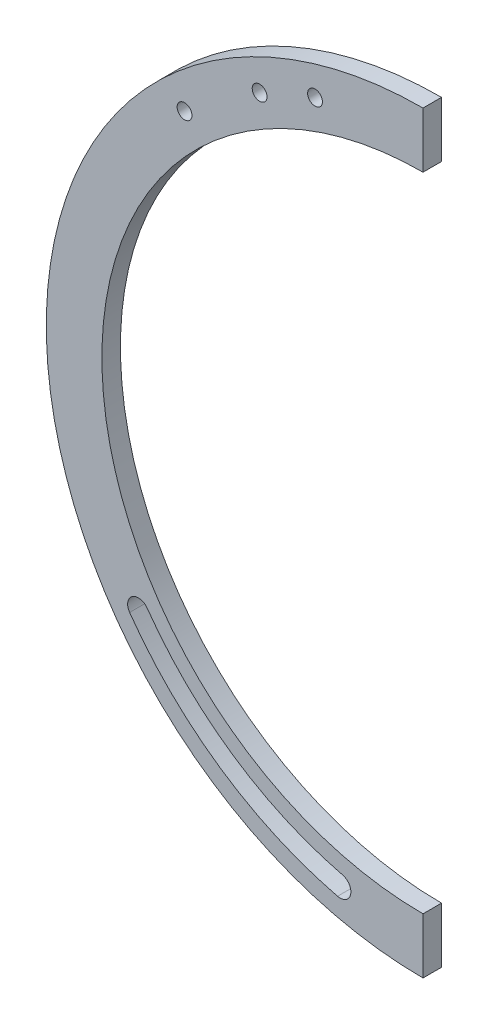
from build123d import *

# Parameters (mm, degrees)
SKETCH1_R               = 203.294925519
SKETCH1_R_2             = 173.294925519
BOSS_EXTRUDE1_DEPTH     = 10
CUT_EXTRUDE1_START      = -185
CUT_EXTRUDE1_DEPTH      = 185
CUT_EXTRUDE2_DEPTH      = 185
CUT_EXTRUDE3_DEPTH      = 484.877792972
CUT_EXTRUDE3_DEPTH_BACK = 484.877792972
SKETCH4_R               = 4


with BuildPart() as part:
    # Sketch1 → Boss-Extrude1 (new body)
    with BuildSketch(Plane.XY):
        with Locations((291.585214163, 182.730697222)):
            Circle(SKETCH1_R)
        with Locations((291.585214163, 182.730697222)):
            Circle(SKETCH1_R_2, mode=Mode.SUBTRACT)
    extrude(amount=-BOSS_EXTRUDE1_DEPTH)

    # Sketch2 → Cut-Extrude1 (cut)
    with BuildSketch(Plane(origin=(0, 0, -10), x_dir=(-1, 0, 0), z_dir=(0, 0, -1)).offset(CUT_EXTRUDE1_START)):
        with BuildLine():
            Line((-291.585214163, 9.435771703), (-291.585214163, -33.905509081))
            ThreePointArc((-291.585214163, -33.905509081), (-508.221420466, 182.730697222), (-291.585214163, 399.366903525))
            Line((-291.585214163, 399.366903525), (-291.585214163, 356.025622742))
            ThreePointArc((-291.585214163, 356.025622742), (-464.880139683, 182.730697222), (-291.585214163, 9.435771703))
        make_face()
    extrude(amount=CUT_EXTRUDE1_DEPTH, mode=Mode.SUBTRACT)

    # Sketch3 → Cut-Extrude2 (cut)
    with BuildSketch(Plane(origin=(0, 0, -10), x_dir=(-1, 0, 0), z_dir=(0, 0, -1))):
        with BuildLine():
            ThreePointArc((-245.463287057, -5.419646314), (-182.427275621, 22.692175653), (-133.247878722, 71.11944269))
            ThreePointArc((-133.247878722, 71.11944269), (-134.651744503, 79.229936459), (-142.762238272, 77.826070678))
            ThreePointArc((-142.762238272, 77.826070678), (-188.98648588, 32.30875807), (-248.234715516, 5.886152238))
            ThreePointArc((-248.234715516, 5.886152238), (-252.501900562, -1.152461267), (-245.463287057, -5.419646314))
        make_face()
    extrude(amount=-CUT_EXTRUDE2_DEPTH, mode=Mode.SUBTRACT)

    # Sketch4 → Cut-Extrude3 (cut, two sides: drawn at the far end of the back side and taken through both)
    with BuildSketch(Plane(origin=(0, 0, -10), x_dir=(-1, 0, 0), z_dir=(0, 0, -1)).offset(-CUT_EXTRUDE3_DEPTH_BACK)):
        with Locations((-203.411601384, 349.104953001)):
            Circle(SKETCH4_R)
        with Locations((-233.317748738, 361.783430933)):
            Circle(SKETCH4_R)
        with Locations((-162.898022452, 320.188274917)):
            Circle(SKETCH4_R)
    extrude(amount=CUT_EXTRUDE3_DEPTH + CUT_EXTRUDE3_DEPTH_BACK, mode=Mode.SUBTRACT)


solid = part.part
